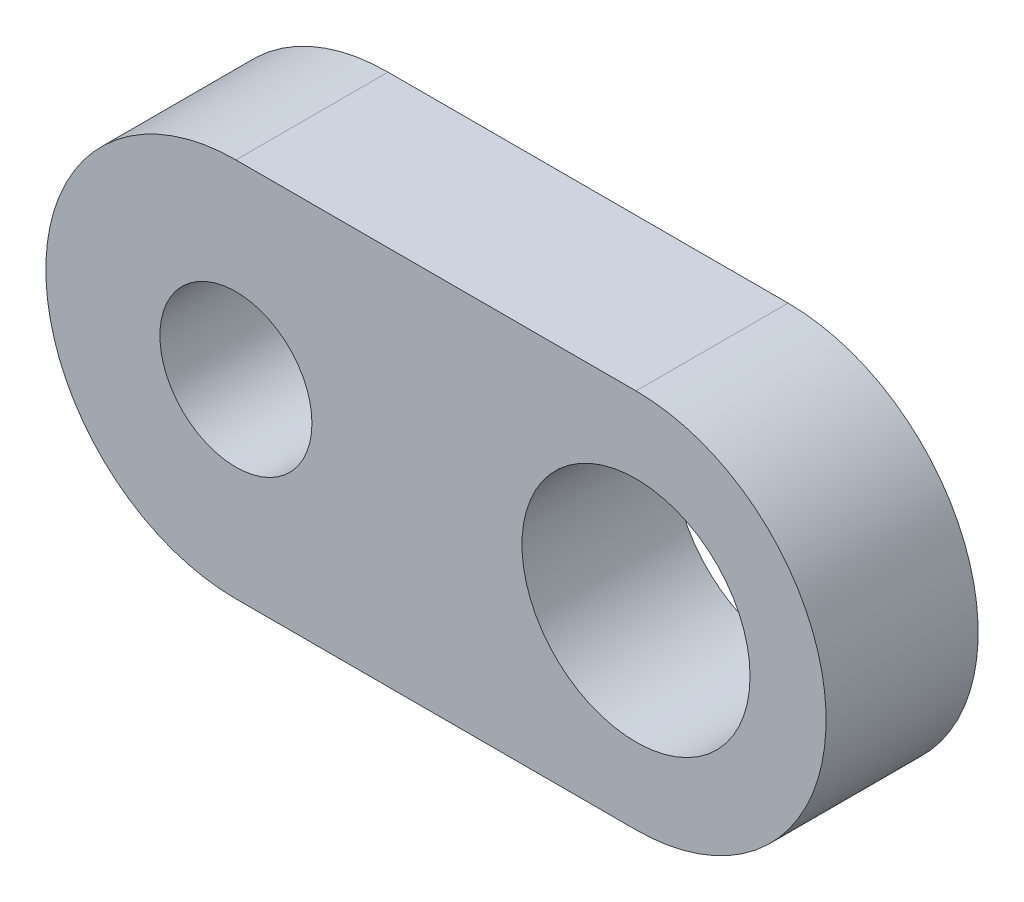
SolidWorks part; units mm, degrees
material "1060 合金"
ref_plane "前视基准面" through (0, 0, 0) normal (0, 0, 1) x (1, 0, 0)
ref_plane "上视基准面" through (0, 0, 0) normal (0, 1, 0) x (1, 0, 0)
ref_plane "右视基准面" through (0, 0, 0) normal (1, 0, 0) x (0, 0, -1)
sketch "草图1" plane through (0, 0, 0) normal (0, 0, 1) x (1, 0, 0)
  line L0 (-13.155, 0) -> (13.155, 0) construction
  line L1 (-13.155, 12.5) -> (13.155, 12.5)
  line L2 (-13.155, -12.5) -> (13.155, -12.5)
  arc A0 (-13.155, 12.5) -> (-13.155, -12.5) centre (-13.155, 0) ccw
  arc A1 (13.155, -12.5) -> (13.155, 12.5) centre (13.155, 0) ccw
  circle A3 centre (13.155, 0) radius 7.5
  circle A4 centre (-13.155, 0) radius 5
  point P2 (0, 0)
  dimension "D3" = 10
  dimension "D4" = 15
  dimension "D1" = 25
  dimension "D2" = 26.31
extrude "凸台-拉伸1" add sketch "草图1" along normal blind 10
